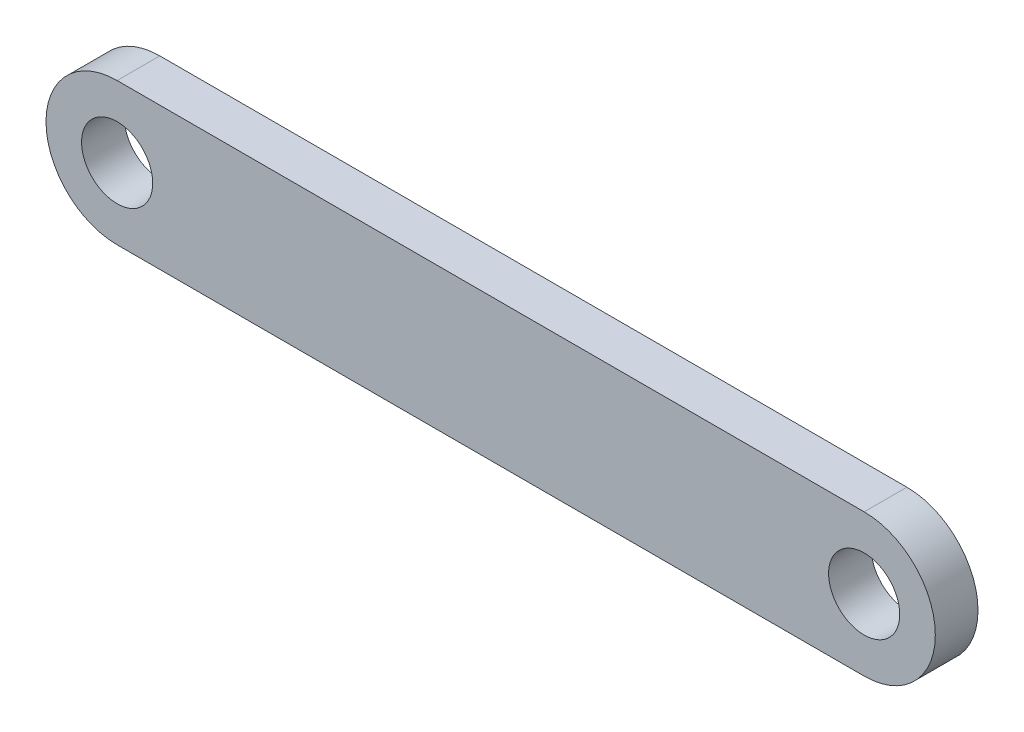
from build123d import *

# Parameters (mm, degrees)
SKETCH1_R           = 5
BOSS_EXTRUDE1_DEPTH = 3


with BuildPart() as part:
    # Sketch1 → Boss-Extrude1 (new, symmetric)
    with BuildSketch(Plane.XY):
        with BuildLine():
            Line((0, 10), (105, 10))
            ThreePointArc((105, 10), (115, 0), (105, -10))
            Line((105, -10), (0, -10))
            ThreePointArc((0, -10), (-10, 0), (0, 10))
        make_face()
        Circle(SKETCH1_R, mode=Mode.SUBTRACT)
        with Locations((105, 0)):
            Circle(SKETCH1_R, mode=Mode.SUBTRACT)
    extrude(amount=BOSS_EXTRUDE1_DEPTH, both=True)


solid = part.part
